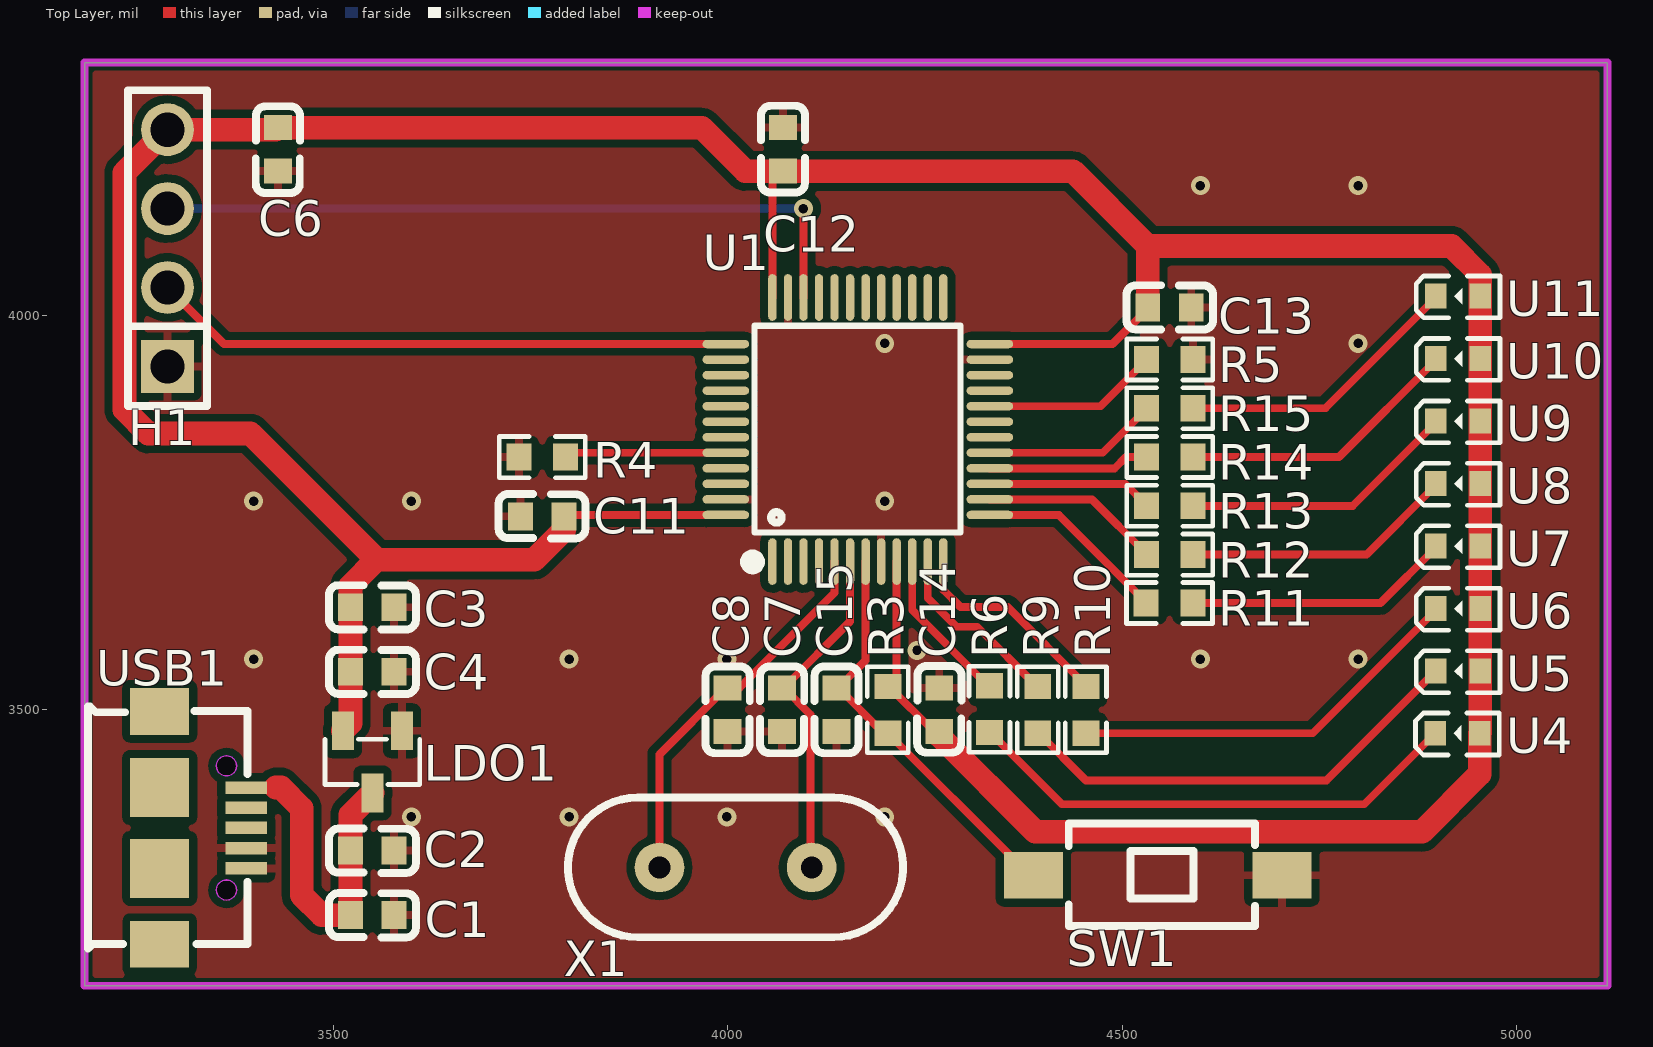
[diagram p0: Top Layer view]
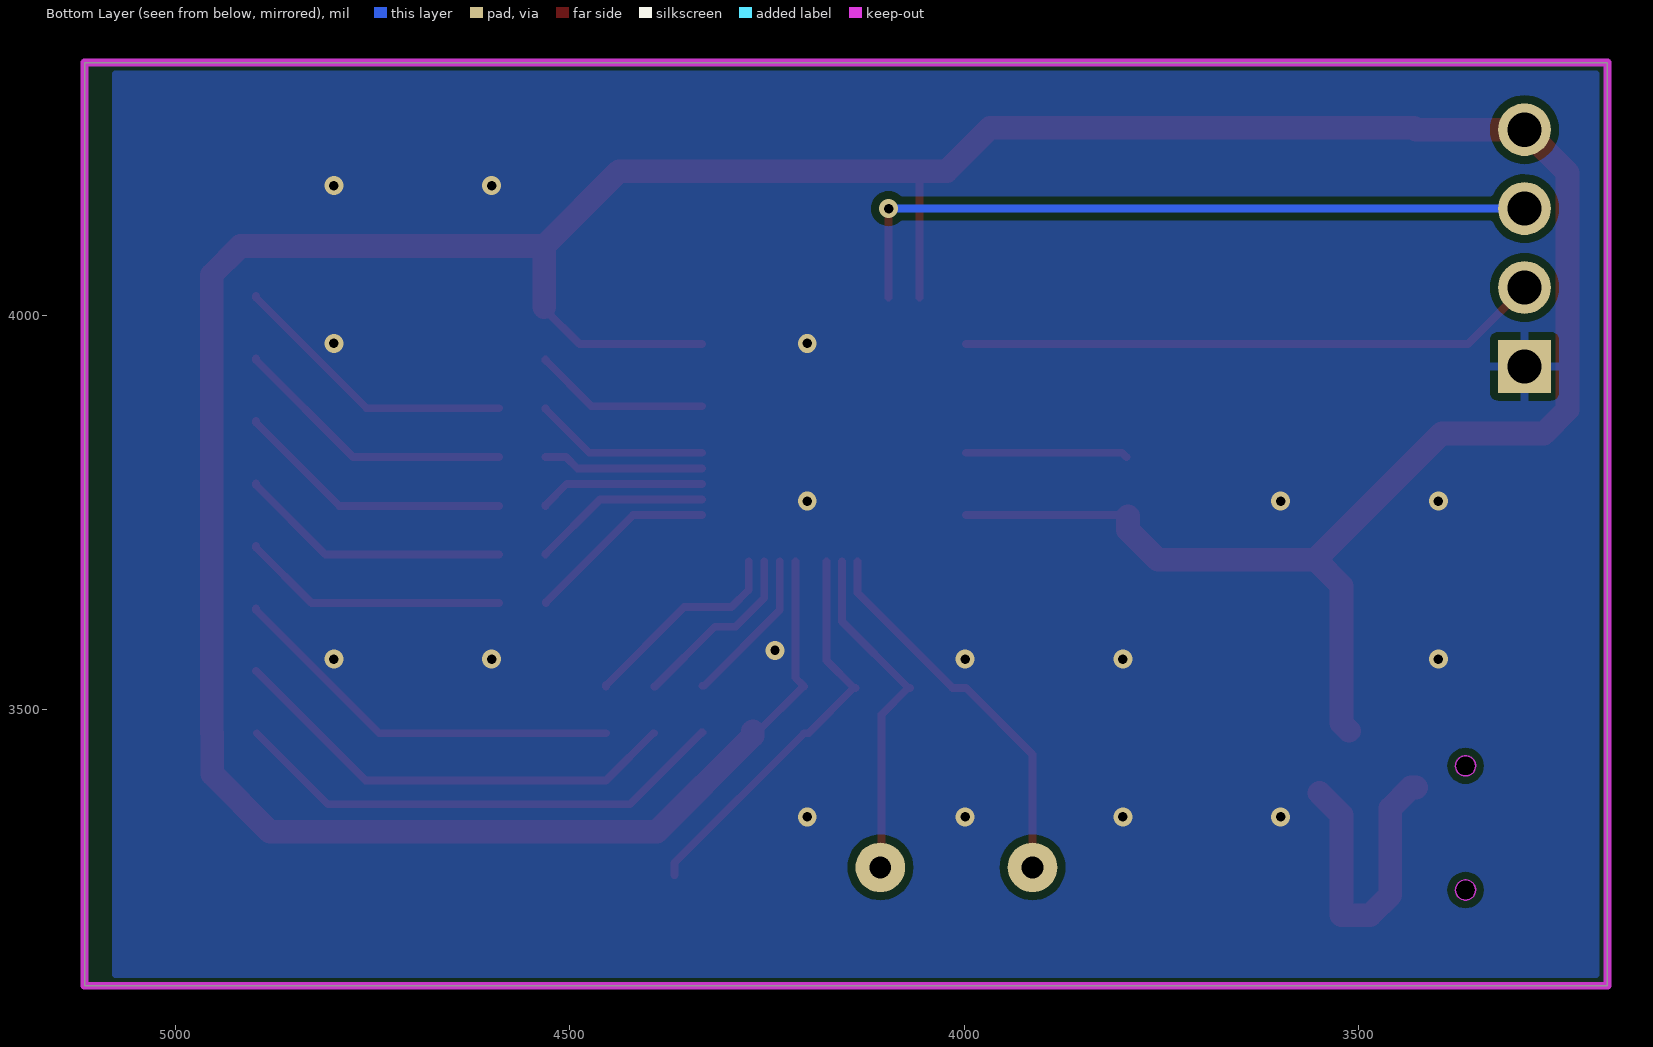
[diagram p1: Bottom Layer view, seen from below]
# Altium PCB MISC61263.pcbdoc
Units mil, origin at the board's own origin, x right, y up, seen from the top; angles counter-clockwise.
Board outline 1930 x 1170 mil, 2 copper layers (Top Layer, Bottom Layer), stack 62.206 mil thick; 37 components, 51 nets, 130 pads, 18 vias.

## Layer stack, top to bottom
Top Solder Mask Layer: solder mask 0.394, Dk 3.3
Top Layer: signal copper 1.379
Dielectric1: surface 59.449, FR4, Dk 4.5
Bottom Layer: signal copper 1.378
Bottom Solder Mask Layer: solder mask 0.394, Dk 3.3

## Board outline
3185,4320 3185,3150 5115,3150 5115,4320

## Design rules (kind name [scope] priority, off if disabled: settings)
BoardOutlineClearance copperThickness2oz_1 [All] p2 off: genericclearance=7.99 ignorepadtopadclearanceinfootprint=FALSE except(0: Arc-SplitContinuation Track-SplitContinuation SMDPad-SplitContinuation THPad-SplitContinuation Via-SplitContinuation Fill-SplitContinuation Region-SplitContinuation Poly-SplitContinuation Text-SplitContinuation Hole-SplitContinuation; 5.98: SMDPad-CutoutEdge THPad-CutoutEdge Via-CutoutEdge Fill-CutoutEdge Region-CutoutEdge Text-CutoutEdge Hole-CutoutEdge; 10: Poly-OutlineEdge Poly-CutoutEdge; 11.81: Arc-OutlineEdge Track-OutlineEdge SMDPad-OutlineEdge THPad-OutlineEdge Via-OutlineEdge Fill-OutlineEdge Region-OutlineEdge Text-OutlineEdge Hole-OutlineEdge Arc-CutoutEdge Track-CutoutEdge)
BoardOutlineClearance Plane_innerPlane_1 [All] p4 off: genericclearance=4.02 ignorepadtopadclearanceinfootprint=FALSE except(0: Arc-SplitContinuation Track-SplitContinuation SMDPad-SplitContinuation THPad-SplitContinuation Via-SplitContinuation Fill-SplitContinuation Region-SplitContinuation Poly-SplitContinuation Text-SplitContinuation Hole-SplitContinuation; 5.98: SMDPad-CutoutEdge THPad-CutoutEdge Via-CutoutEdge Fill-CutoutEdge Region-CutoutEdge Text-CutoutEdge Hole-CutoutEdge; 10: Poly-OutlineEdge Poly-CutoutEdge; 11.81: Arc-OutlineEdge Track-OutlineEdge SMDPad-OutlineEdge THPad-OutlineEdge Via-OutlineEdge Fill-OutlineEdge Region-OutlineEdge Text-OutlineEdge Hole-OutlineEdge Arc-CutoutEdge Track-CutoutEdge)
BoardOutlineClearance Copper_copperRegion_1 [All] p6 off: genericclearance=4.02 ignorepadtopadclearanceinfootprint=FALSE except(0: Arc-SplitContinuation Track-SplitContinuation SMDPad-SplitContinuation THPad-SplitContinuation Via-SplitContinuation Fill-SplitContinuation Region-SplitContinuation Poly-SplitContinuation Text-SplitContinuation Hole-SplitContinuation; 5.98: SMDPad-CutoutEdge THPad-CutoutEdge Via-CutoutEdge Fill-CutoutEdge Region-CutoutEdge Text-CutoutEdge Hole-CutoutEdge; 10: Poly-OutlineEdge Poly-CutoutEdge; 11.81: Arc-OutlineEdge Track-OutlineEdge SMDPad-OutlineEdge THPad-OutlineEdge Via-OutlineEdge Fill-OutlineEdge Region-OutlineEdge Text-OutlineEdge Hole-OutlineEdge Arc-CutoutEdge Track-CutoutEdge)
BoardOutlineClearance copperThickness1oz_1 [All] p8: genericclearance=4.02 ignorepadtopadclearanceinfootprint=FALSE except(0: Arc-SplitContinuation Track-SplitContinuation SMDPad-SplitContinuation THPad-SplitContinuation Via-SplitContinuation Fill-SplitContinuation Region-SplitContinuation Poly-SplitContinuation Text-SplitContinuation Hole-SplitContinuation; 5.98: SMDPad-CutoutEdge THPad-CutoutEdge Via-CutoutEdge Fill-CutoutEdge Region-CutoutEdge Text-CutoutEdge Hole-CutoutEdge; 10: Poly-OutlineEdge Poly-CutoutEdge; 11.81: Arc-OutlineEdge Track-OutlineEdge SMDPad-OutlineEdge THPad-OutlineEdge Via-OutlineEdge Fill-OutlineEdge Region-OutlineEdge Text-OutlineEdge Hole-OutlineEdge Arc-CutoutEdge Track-CutoutEdge)
Clearance copperThickness2oz [All] p1 off: gap=7.99 ignorepadtopadclearanceinfootprint=FALSE except(5.98: SMDPad-Track SMDPad-SMDPad THPad-Track SMDPad-THPad THPad-THPad Track-Via SMDPad-Via THPad-Via Via-Via Fill-Track Region-Track Fill-SMDPad Region-SMDPad Fill-THPad Region-THPad Fill-Via Region-Via Fill-Fill Fill-Region Region-Region Arc-Track Arc-SMDPad Arc-THPad Arc-Via Fill-Arc Region-Arc Arc-Arc Text-Track SMDPad-Text Text-THPad Text-Via Fill-Text Region-Text Arc-Text Text-Text Hole-Track Hole-SMDPad Hole-THPad Hole-Via Fill-Hole Region-Hole Hole-Arc Hole-Text; 10: Poly-Track Poly-SMDPad Poly-THPad Poly-Via Poly-Fill Poly-Region Poly-Poly Poly-Arc Poly-Text Poly-Hole)
Clearance Plane_innerPlane [All] p3 off: gap=4.02 ignorepadtopadclearanceinfootprint=FALSE except(5.98: SMDPad-Track SMDPad-SMDPad THPad-Track SMDPad-THPad THPad-THPad Track-Via SMDPad-Via THPad-Via Via-Via Fill-Track Region-Track Fill-SMDPad Region-SMDPad Fill-THPad Region-THPad Fill-Via Region-Via Fill-Fill Fill-Region Region-Region Arc-Track Arc-SMDPad Arc-THPad Arc-Via Fill-Arc Region-Arc Arc-Arc Text-Track SMDPad-Text Text-THPad Text-Via Fill-Text Region-Text Arc-Text Text-Text Hole-Track Hole-SMDPad Hole-THPad Hole-Via Fill-Hole Region-Hole Hole-Arc Hole-Text; 10: Poly-Track Poly-SMDPad Poly-THPad Poly-Via Poly-Fill Poly-Region Poly-Poly Poly-Arc Poly-Text Poly-Hole)
Clearance Copper_copperRegion [All] p5 off: gap=4.02 ignorepadtopadclearanceinfootprint=FALSE except(5.98: SMDPad-Track SMDPad-SMDPad THPad-Track SMDPad-THPad THPad-THPad Track-Via SMDPad-Via THPad-Via Via-Via Fill-Track Region-Track Fill-SMDPad Region-SMDPad Fill-THPad Region-THPad Fill-Via Region-Via Fill-Fill Fill-Region Region-Region Arc-Track Arc-SMDPad Arc-THPad Arc-Via Fill-Arc Region-Arc Arc-Arc Text-Track SMDPad-Text Text-THPad Text-Via Fill-Text Region-Text Arc-Text Text-Text Hole-Track Hole-SMDPad Hole-THPad Hole-Via Fill-Hole Region-Hole Hole-Arc Hole-Text; 10: Poly-Track Poly-SMDPad Poly-THPad Poly-Via Poly-Fill Poly-Region Poly-Poly Poly-Arc Poly-Text Poly-Hole)
Clearance copperThickness1oz [All] p7: gap=4.02 ignorepadtopadclearanceinfootprint=FALSE except(5.98: SMDPad-Track SMDPad-SMDPad THPad-Track SMDPad-THPad THPad-THPad Track-Via SMDPad-Via THPad-Via Via-Via Fill-Track Region-Track Fill-SMDPad Region-SMDPad Fill-THPad Region-THPad Fill-Via Region-Via Fill-Fill Fill-Region Region-Region Arc-Track Arc-SMDPad Arc-THPad Arc-Via Fill-Arc Region-Arc Arc-Arc Text-Track SMDPad-Text Text-THPad Text-Via Fill-Text Region-Text Arc-Text Text-Text Hole-Track Hole-SMDPad Hole-THPad Hole-Via Fill-Hole Region-Hole Hole-Arc Hole-Text; 10: Poly-Track Poly-SMDPad Poly-THPad Poly-Via Poly-Fill Poly-Region Poly-Poly Poly-Arc Poly-Text Poly-Hole)
DiffPairsRouting differentialPair [All] p1: maxlimit=6 minlimit=6 mostfreqgap=6 toplayer_minwidth=5 toplayer_prefwidth=10 toplayer_maxwidth=100 toplayer_mingap=6 toplayer_prefgap=6 toplayer_maxgap=6 bottomlayer_minwidth=5 bottomlayer_prefwidth=10 bottomlayer_maxwidth=100 bottomlayer_mingap=6 bottomlayer_prefgap=6 bottomlayer_maxgap=6 maxuncoupledlength=10
HoleToHoleClearance otherClearance [All] p1: gap=11.8 allowstackedmicrovias=TRUE
Length netLength [All] p1: minlimit=0 maxlimit=0
PasteMaskExpansion pasteMaskExpansion [All] p1: expansion=0
PlaneConnect innerPlane [All] p1: planeconnectstyle=Relief reliefexpansion=20 reliefentries=4 reliefconductorwidth=10 reliefairgap=10
PolygonConnect copperRegion [All] p1: connectstyle=Relief reliefconductorwidth=10 reliefentries=4 polygonreliefangle="90 Angle" airgapwidth=10 via.connectstyle=Relief via.reliefconductorwidth=10 via.reliefentries=4 via.polygonreliefangle="90 Angle" via.airgapwidth=10
RoutingVias viaSize [All] p1: holewidth=12.01 width=24.02 viastyle="Through Hole" minholewidth=11.81 minwidth=19.68 maxholewidth=248.03 maxwidth=393.7
SolderMaskExpansion solderMaskExpansion [IsVia] p1: expansion=-1000 istentingtop=TRUE
SolderMaskExpansion solderMaskExpansion [All] p2: expansion=2 istentingtop=FALSE
Width copperThickness2oz_2 [All] p1 off: maxlimit=100 minlimit=8 preferedwidth=10
Width copperThickness1oz_2 [All] p2: maxlimit=100 minlimit=5 preferedwidth=10

## Components (designator, comment, footprint, x,y, rotation, side; value= is the part's Value field where it differs from the comment)
C1 "10uF" C0603 3549.49,3239.5 r180 top
C2 "100nF" C0603 3549.49,3321.24 r180 top
C3 "100nF" C0603 3549.49,3629.69 r180 top
C4 "10uF" C0603 3549.49,3547.95 r180 top
C6 "100nF" C0603 3430,4210 r90 top
C7 "20pF" C0603 4069.07,3500 r90 top
C8 "20pF" C0603 4000,3500 r90 top
C11 "100nF" C0603 3765,3745 r0 top
C12 "100nF" C0603 4070,4210 r270 top
C13 "100nF" C0603 4560.05,4009.82 r180 top
C14 "100nF" C0603 4268.17,3500 r270 top
C15 "10uF" C0603 4138.14,3500 r90 top
H1 "" HDR-TH_4P-P2.54-V-M 3290,4085 r90 top
LDO1 "SC662K-3.3V" SOT-23-3_L2.9-W1.3-P1.90-LS2.4-BR 3549.79,3433.8 r90 top
R3 "1kΩ" R0603 4203.04,3499.7 r90 top
R4 "10kΩ" R0603 3765,3820 r0 top
R5 "10kΩ" R0603 4560.35,3943.82 r180 top
R6 "510Ω" R0603 4331.83,3500.54 r90 top
R9 "510Ω" R0603 4393.07,3499.7 r90 top
R10 "510Ω" R0603 4454.04,3499.7 r90 top
R11 "510Ω" R0603 4560,3635 r180 top
R12 "510Ω" R0603 4560.35,3696.43 r180 top
R13 "510Ω" R0603 4560.35,3758.27 r180 top
R14 "510Ω" R0603 4560.35,3820.12 r180 top
R15 "510Ω" R0603 4560.35,3881.97 r180 top
SW1 "TS-1101-C-W" SW-SMD_L6.0-W3.3-LS8.0 4545,3290 r180 top
U1 "STM32F103C8T6" LQFP-48_L7.0-W7.0-P0.50-LS9.0-BL 4165,3855 r0 top
U4 "42-51/GHC-YW2X2K/3T" LED-SMD_L1.6-W0.8-FD_GREEN-1 4925,3470 r180 top
U5 "42-51/GHC-YW2X2K/3T" LED-SMD_L1.6-W0.8-FD_GREEN-1 4925.75,3548.81 r180 top
U6 "42-51/GHC-YW2X2K/3T" LED-SMD_L1.6-W0.8-FD_GREEN-1 4925.75,3628.02 r180 top
U7 "42-51/GHC-YW2X2K/3T" LED-SMD_L1.6-W0.8-FD_GREEN-1 4925.75,3707.22 r180 top
U8 "42-51/GHC-YW2X2K/3T" LED-SMD_L1.6-W0.8-FD_GREEN-1 4925.75,3786.43 r180 top
U9 "42-51/GHC-YW2X2K/3T" LED-SMD_L1.6-W0.8-FD_GREEN-1 4925.75,3865.63 r180 top
U10 "42-51/GHC-YW2X2K/3T" LED-SMD_L1.6-W0.8-FD_GREEN-1 4925.75,3944.84 r180 top
U11 "42-51/GHC-YW2X2K/3T" LED-SMD_L1.6-W0.8-FD_GREEN-1 4925.75,4024.04 r180 top
USB1 "920-D62A2021S10100" MICRO-USB-SMD_5P-P0.65-H-M_MICRO-USB-5P 3335,3350 r270 top
X1 "8MHz" OSC-TH_L10.0-W4.5-P5.00 4010,3300 r90 top

## Footprints (in the part's own frame and the unit in brackets; to place one, negate y for a bottom-side part, rotate by r counter-clockwise, add the part's x,y. Pads: shape width x height; smd on the part's side, far side on the other; paste and mask are expansions set on the pad)
C0603 [mm]
  rect 0.8x0.9 smd: 1(-0.7,0) 2(0.7,0)
  silkscreen extent -1.41,-0.71 1.39,0.72
HDR-TH_4P-P2.54-V-M [mm]
  rect 1.7x1.7 hole 1.1: 1(-3.81,0)
  round 1.7 hole 1.1: 2(-1.27,0) 3(1.27,0) 4(3.81,0)
  silkscreen extent -5.08,-1.27 5.08,1.27
LED-SMD_L1.6-W0.8-FD_GREEN-1 [mm]
  rect 0.7x0.8 smd: 1(-0.715,0) 2(0.715,0)
  silkscreen extent -1.35,-0.65 1.35,0.7
LQFP-48_L7.0-W7.0-P0.50-LS9.0-BL [mm]
  oval 0.27x1.5 smd paste+0 mask+0.05: 1(-2.75,-4.25) 2(-2.25,-4.25) 3(-1.75,-4.25) 4(-1.25,-4.25) 5(-0.75,-4.25) 6(-0.25,-4.25) 7(0.25,-4.25) 8(0.75,-4.25) 9(1.25,-4.25) 10(1.75,-4.25) 11(2.25,-4.25) 12(2.75,-4.25) 25(2.75,4.25) 26(2.25,4.25) 27(1.75,4.25) 28(1.25,4.25) 29(0.75,4.25) 30(0.25,4.25) 31(-0.25,4.25) 32(-0.75,4.25) 33(-1.25,4.25) 34(-1.75,4.25) 35(-2.25,4.25) 36(-2.75,4.25)
  oval 1.5x0.27 smd paste+0 mask+0.05: 13(4.25,-2.75) 14(4.25,-2.25) 15(4.25,-1.75) 16(4.25,-1.25) 17(4.25,-0.75) 18(4.25,-0.25) 19(4.25,0.25) 20(4.25,0.75) 21(4.25,1.25) 22(4.25,1.75) 23(4.25,2.25) 24(4.25,2.75) 37(-4.25,2.75) 38(-4.25,2.25) 39(-4.25,1.75) 40(-4.25,1.25) 41(-4.25,0.75) 42(-4.25,0.25) 43(-4.25,-0.25) 44(-4.25,-0.75) 45(-4.25,-1.25) 46(-4.25,-1.75) 47(-4.25,-2.25) 48(-4.25,-2.75)
  silkscreen extent -3.59,-4.46 3.3,3.34
MICRO-USB-SMD_5P-P0.65-H-M_MICRO-USB-5P [mm]
  rect 1.5x1.9 smd: 0(-3.75,-1.392) 0(3.75,-1.392)
  rect 1.9x1.9 smd: 0(-1.3,-1.392) 0(1.3,-1.392)
  rect 0.4x1.35 smd: 1(-1.3,1.392) 2(-0.65,1.392) 3(0,1.392) 4(0.65,1.392) 5(1.3,1.392)
  Board Outline Layer circle w0.003: c-1.999,0.756 r0.325
  Board Outline Layer circle w0.003: c1.999,0.756 r0.325
  Board Outline Layer region: -1.999,1.081 -1.858,1.049 -1.745,0.959 -1.682,0.829 -1.682,0.684 -1.745,0.554 -1.858,0.464 -1.999,0.431 -1.999,0.431 -2.14,0.464 -2.253,0.554 -2.316,0.684 -2.316,0.829 -2.253,0.959 -2.14,1.049 -1.999,1.081
  Board Outline Layer region: -1.999,1.081 -1.921,1.072 -1.848,1.044 -1.783,1 -1.732,0.941 -1.695,0.872 -1.676,0.796 -1.676,0.717 -1.695,0.641 -1.732,0.572 -1.783,0.513 -1.848,0.469 -1.921,0.441 -1.999,0.431 -2.077,0.441 -2.15,0.469 -2.214,0.513 -2.266,0.572 -2.303,0.641 -2.322,0.717 -2.322,0.796 -2.303,0.872 -2.266,0.941 -2.214,1 -2.15,1.044 -2.077,1.072
  Board Outline Layer region: 1.999,1.081 2.14,1.049 2.253,0.959 2.316,0.829 2.316,0.684 2.253,0.554 2.14,0.464 1.999,0.431 1.999,0.431 1.858,0.464 1.745,0.554 1.682,0.684 1.682,0.829 1.745,0.959 1.858,1.049 1.999,1.081
  Board Outline Layer region: 1.999,1.081 2.077,1.072 2.15,1.044 2.214,1 2.266,0.941 2.303,0.872 2.322,0.796 2.322,0.717 2.303,0.641 2.266,0.572 2.214,0.513 2.15,0.469 2.077,0.441 1.999,0.431 1.921,0.441 1.848,0.469 1.783,0.513 1.732,0.572 1.695,0.641 1.676,0.717 1.676,0.796 1.695,0.872 1.732,0.941 1.783,1 1.848,1.044 1.921,1.072
  Multi-Layer board cut-out: -1.999,1.081 -1.858,1.049 -1.745,0.959 -1.682,0.829 -1.682,0.684 -1.745,0.554 -1.858,0.464 -1.999,0.431 -1.999,0.431 -2.14,0.464 -2.253,0.554 -2.316,0.684 -2.316,0.829 -2.253,0.959 -2.14,1.049 -1.999,1.081
  Multi-Layer board cut-out: 1.999,1.081 2.14,1.049 2.253,0.959 2.316,0.829 2.316,0.684 2.253,0.554 2.14,0.464 1.999,0.431 1.999,0.431 1.858,0.464 1.745,0.554 1.682,0.684 1.682,0.829 1.745,0.959 1.858,1.049 1.999,1.081
  silkscreen extent -3.91,-3.7 3.88,1.43
OSC-TH_L10.0-W4.5-P5.00 [mm]
  round 1.6 hole 0.7: 1(0,2.45) 2(0,-2.45)
  silkscreen extent -2.25,-5.39 2.25,5.39
R0603 [mil]
  rect 31.75x34.02 smd paste-3937.01 mask+2: 1(-29.66,0) 2(29.66,0)
  silkscreen extent -55,-26 55,26
SOT-23-3_L2.9-W1.3-P1.90-LS2.4-BR [mm]
  rect 1.25x0.7 smd: 1(1,-0.95) 2(1,0.95) 3(-1,0)
  silkscreen extent -0.73,-1.53 0.73,1.53
SW-SMD_L6.0-W3.3-LS8.0 [mm]
  rect 1.9x1.5 smd: 1(-4,0) 2(4,0)
  silkscreen extent -3.14,-1.67 2.86,1.63

## Via types
v1: diameter 24.02, hole 12, Top Layer to Bottom Layer, 18 vias

## Nets (pads, with @x,y where several pads share a name; then routed paths per layer and width w, separated by ;. In a path a pad name is that pad's centre, name@x,y a point inside that pad or via, vN(x,y) a via of type N, cw(c..) or ccw(c..) an arc to the next point about the centre after c; other vN are vias at no path point)
3V3: C3.2 C4.2 C6.2 C11.2 C12.2 C13.2 C14.2 H1.4 LDO1.2 R3.2 U1.9 U1.24 U1.36 U1.48 U4.1 U5.1 U6.1 U7.1 U8.1 U9.1 U10.1 U11.1 | length 5347
  Top Layer w10: C11.2 3794.29,3746.73 U1.48 ; U1.36 4056.73,4169.17 C12.2 ; U1.9 4214.21,3540.52 R3.2 4204.18,3529.36 4261.09,3472.44 C14.2 ; U1.24 4487.9,3963.27 C13.2@4532.49,4007.85
  Top Layer w30: LDO1.2 3521.93,3482.7 C4.2 C3.2 3521.93,3656.93 3555,3690 ; C11.2 3792.56,3727.56 3755,3690 3555,3690 ; C14.2 4268.17,3466.83 4390,3345 4880,3345 4953.15,3418.15 U4.1 4953.9,3470.75 U5.1 U6.1 U7.1 U8.1 U9.1 U10.1 U11.1 4953.9,4051.1 4917.49,4087.51 4532.49,4087.51 ; C13.2 4532.49,4087.51 ; 3555,3690 3395,3850 3265.55,3850 3235.55,3880 3235.55,4180.55 H1.4 3427.44,4235 C6.2 3967.16,4237.56 4022.28,4182.44 C12.2 4437.56,4182.44 4532.49,4087.51
$1N5662: R6.1 U4.2 | length 639.9
  Top Layer w10: R6.1 4332.96,3470.88 4423.85,3380 4806.85,3380 U4.2
$1N14583: R9.1 U5.2 | length 586.9
  Top Layer w10: R9.1 4394.21,3470.03 4454.24,3410 4758.79,3410 U5.2
$1N14664: R10.1 U6.2 | length 510.2
  Top Layer w10: R10.1 4741.58,3470.03 4897.6,3626.05 U6.2
$1N14747: R11.1 U7.2 | length 339
  Top Layer w10: R11.1 4827.34,3635 4897.6,3705.25 U7.2
$1N14822: R12.1 U8.2 | length 346
  Top Layer w10: R12.1 4809.57,3696.43 4897.6,3784.46 U8.2
$1N14897: R13.1 U9.2 | length 353.2
  Top Layer w10: R13.1 4792.21,3758.27 4897.6,3863.66 U9.2
$1N14972: R14.1 U10.2 | length 360.4
  Top Layer w10: R14.1 4774.85,3820.12 4897.6,3942.87 U10.2
$1N15047: R15.1 U11.2 | length 367.6
  Top Layer w10: R15.1 4757.49,3881.97 4897.6,4022.07 U11.2
+5V: C1.2 C2.2 LDO1.3 USB1.1 | length 392.2
  Top Layer w30: 3427.63,3401.2 3433.8,3401.2 3460,3375 3460,3265 3485.5,3239.5 C1.2 C2.2 3521.93,3366.56 LDO1.3
BOOT0: R4.2 U1.44 | length 205.3
  Top Layer w10: R4.2 3800.13,3825.47 U1.44
BOOT1: R5.2 U1.20 | length 223.6
  Top Layer w10: U1.20 4472.54,3884.53 4530.69,3942.68 R5.2
CLK: H1.2 U1.37 | length 737.4
  Top Layer w10: H1.2 3361.73,3963.27 U1.37
DIO: H1.3 U1.34 | length 918.8
  Top Layer w10: U1.34 v1(4096.1,4135)
  Bottom Layer w10: H1.3 v1(4096.1,4135)
GND: C1.1 C2.1 C3.1 C4.1 C6.1 C7.1 C8.1 C11.1 C12.1 C13.1 C14.1 C15.1 H1.1 LDO1.1 R4.1 R5.1 SW1.1 U1.8 U1.23 U1.35 U1.47 USB1.4 USB1.5
  other v1: 3599.1,3364.1 3799.1,3364.1 3999.1,3364.1 4199.1,3364.1 3399.1,3564.1 3799.1,3564.1 3999.1,3564.1 4599.1,3564.1 4799.1,3564.1 4240,3575 3399.1,3764.1 3599.1,3764.1 4199.1,3764.1 4199.1,3964.1 4799.1,3964.1 4599.1,4164.1 4799.1,4164.1
OSC32-IN: U1.3
OSC32-OUT: U1.4
OSC-IN: C8.2 U1.5 X1.1 | length 489.5
  Top Layer w10: X1.1 3913.54,3443.07 3998.03,3527.56 C8.2 4014.88,3527.56 4135.47,3648.15 U1.5
OSC-OUT: C7.2 U1.6 X1.2 | length 439.2
  Top Layer w10: C7.2 C7.2@4071.04,3527.56 ; X1.2 4105,3301.46 4105,3493.6 C7.2@4071.04,3527.56 ; U1.6 4155.16,3611.68 C7.2@4071.04,3527.56
PA0: R6.2 U1.10 | length 199.2
  Top Layer w10: U1.10 4233.9,3626.1 4329.8,3530.2 R6.2
PA1: R9.2 U1.11 | length 232.2
  Top Layer w10: U1.11 4253.58,3641.42 4290,3605 4316.3,3605 4391.94,3529.36 R9.2
PA2: R10.2 U1.12 | length 268.3
  Top Layer w10: U1.12 4273.27,3651.73 4295,3630 4355,3630 4454.04,3530.96 R10.2
PA3: R11.2 U1.13 | length 245
  Top Layer w10: U1.13 4419.74,3746.73 4530.34,3636.13 R11.2
PA4: R12.2 U1.14 | length 228
  Top Layer w10: U1.14 4461.83,3766.42 4530.69,3697.56 R12.2
PA5: R13.2 U1.15 | length 210.6
  Top Layer w10: U1.15 4504,3786.1 4530.69,3759.41 R13.2
PA6: R14.2 U1.16 | length 204.3
  Top Layer w10: U1.16 4490.48,3805.79 4504.82,3820.12 R14.2
PA7: R15.2 U1.17 | length 222.4
  Top Layer w10: U1.17 4475.33,3825.47 4530.69,3880.84 R15.2
PA8: U1.29
PA9: U1.30
PA10: U1.31
PA11: U1.32
PA12: U1.33
PA15: U1.38
PB0: U1.18
PB1: U1.19
PB3: U1.39
PB4: U1.40
PB5: U1.41
PB6: U1.42
PB7: U1.43
PB8: U1.45
PB9: U1.46
PB10: U1.21
PB11: U1.22
PB12: U1.25
PB13: U1.26
PB14: U1.27
PB15: U1.28
PC13: U1.2
REST: C15.2 R3.1 SW1.2 U1.7 | length 511.4
  Top Layer w10: C15.2 C15.2@4140.1,3527.56 ; U1.7 4174.84,3562.3 C15.2@4140.1,3527.56 ; SW1.2@4367.52,3290 4367.52,3305.56 R3.1 4197.63,3470.03 C15.2@4140.1,3527.56
VBAT: U1.1
pads on no net: USB1.0 USB1.2 USB1.3

## Polygon pours and split planes (outlines as drawn)
GND on Top Layer (solid, remove dead copper, pour order 0): 3000,4435 3000,3000 5180,3000 5180,4435
GND on Bottom Layer (solid, remove dead copper, pour order 2): 3085,4520 3085,3030 5080,3030 5080,4520

## Keep-outs
Board Outline Layer:
  the board outline again, w10